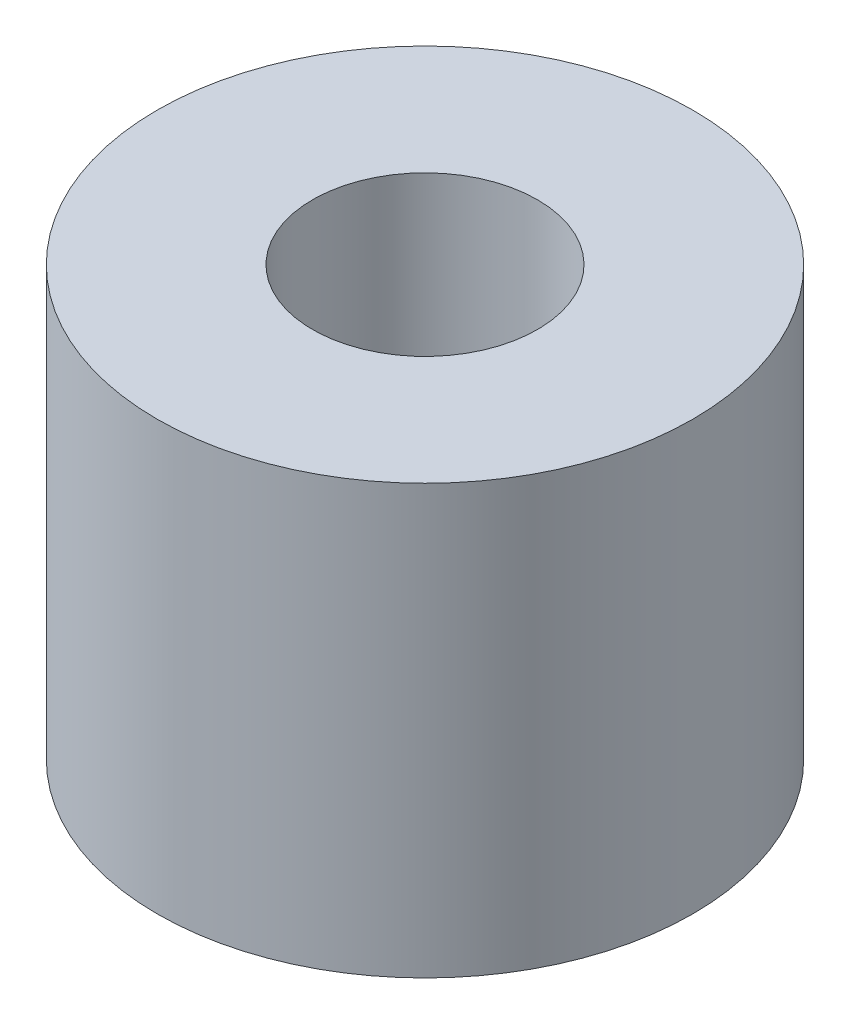
from build123d import *

# Parameters (mm, degrees)
SKETCH1_R                    = 25
BOSS_EXTRUDE1_DEPTH          = 40
M24_TAPPED_HOLE1_D           = 21
M24_TAPPED_HOLE1_CSINK_D     = 24.05
M24_TAPPED_HOLE1_CSINK_ANGLE = 90


with BuildPart() as part:
    # Sketch1 → Boss-Extrude1 (new body)
    with BuildSketch(Plane(origin=(0, 0, 0), x_dir=(1, 0, 0), z_dir=(0, 1, 0))):
        with Locations(Location((0, 0, 0), (0, 0, 270))):
            Circle(SKETCH1_R)
    extrude(amount=BOSS_EXTRUDE1_DEPTH)

    # M24 Tapped Hole1 (through all)
    with Locations(Plane(origin=(0, 0, 0), x_dir=(-1, 0, 0), z_dir=(0, -1, 0))):
        with Locations((0, 0)):
            CounterSinkHole(M24_TAPPED_HOLE1_D / 2, M24_TAPPED_HOLE1_CSINK_D / 2, counter_sink_angle=M24_TAPPED_HOLE1_CSINK_ANGLE)


solid = part.part
